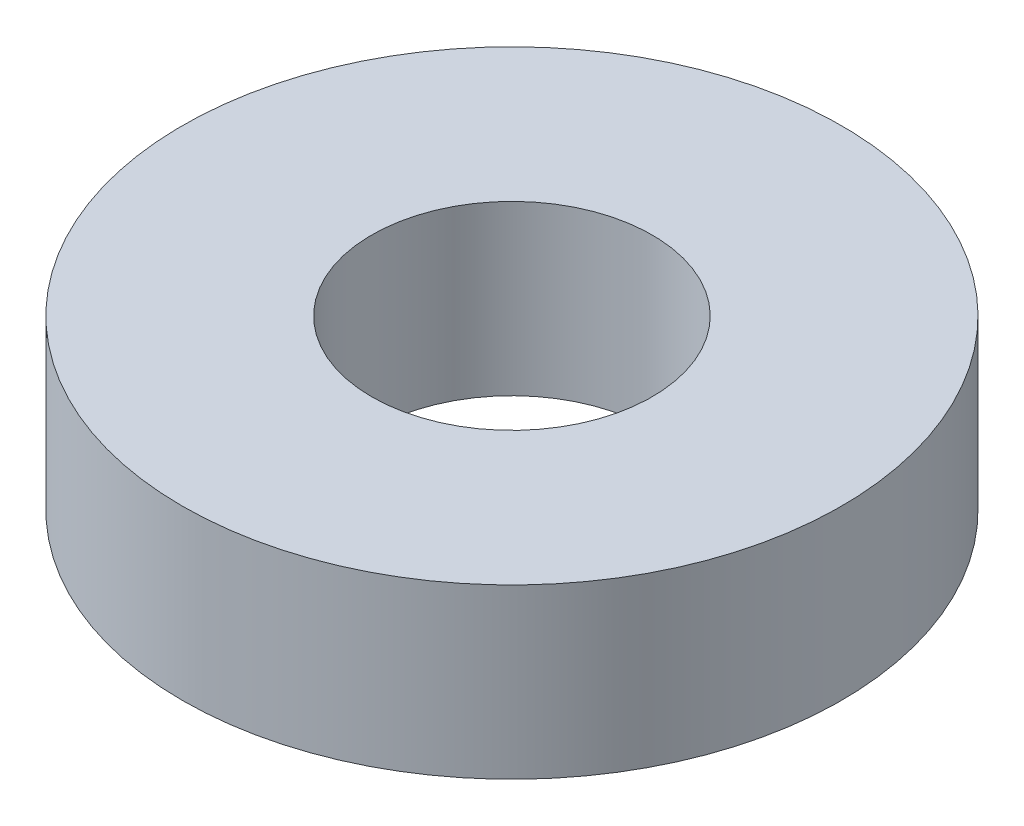
from build123d import *

# Parameters (mm, degrees)
SKETCH1_R           = 23.5
SKETCH1_R_2         = 10
BOSS_EXTRUDE1_DEPTH = 12


with BuildPart() as part:
    # Sketch1 → Boss-Extrude1 (new body)
    with BuildSketch(Plane(origin=(0, 0, 0), x_dir=(1, 0, 0), z_dir=(0, 1, 0))):
        with Locations(Location((0, 0, 0), (0, 0, 270))):
            Circle(SKETCH1_R)
        with Locations(Location((0, 0, 0), (0, 0, 270))):
            Circle(SKETCH1_R_2, mode=Mode.SUBTRACT)
    extrude(amount=BOSS_EXTRUDE1_DEPTH)


solid = part.part
